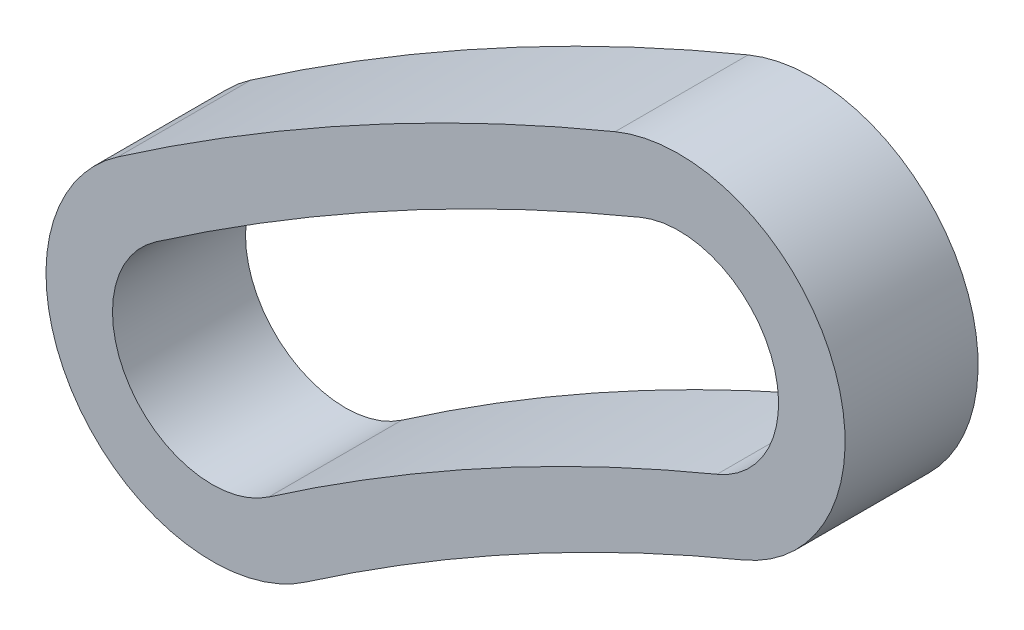
from build123d import *

# Parameters (mm, degrees)
BOSS_EXTRUDE1_DEPTH = 10


with BuildPart() as part:
    # Sketch2 → Boss-Extrude1 (new body)
    with BuildSketch(Plane.XY):
        with BuildLine():
            ThreePointArc((-369.098999305, 369.807855403), (-388.32594275, 360.628087401), (-406.481956169, 349.478976603))
            ThreePointArc((-406.481956169, 349.478976603), (-409.682668352, 332.093481456), (-392.297173205, 328.892769272))
            ThreePointArc((-392.297173205, 328.892769272), (-376.382642925, 338.665446638), (-359.529396201, 346.711909949))
            ThreePointArc((-359.529396201, 346.711909949), (-352.766225026, 363.044684228), (-369.098999305, 369.807855403))
        make_face()
        with BuildLine():
            ThreePointArc((-367.185078684, 365.188666312), (-385.937282785, 356.235559249), (-403.644999576, 345.361735137))
            ThreePointArc((-403.644999576, 345.361735137), (-405.565426886, 334.930438049), (-395.134129798, 333.010010739))
            ThreePointArc((-395.134129798, 333.010010739), (-378.77130289, 343.057974791), (-361.443316822, 351.33109904))
            ThreePointArc((-361.443316822, 351.33109904), (-357.385414117, 361.130763607), (-367.185078684, 365.188666312))
        make_face(mode=Mode.SUBTRACT)
    extrude(amount=BOSS_EXTRUDE1_DEPTH)


solid = part.part
